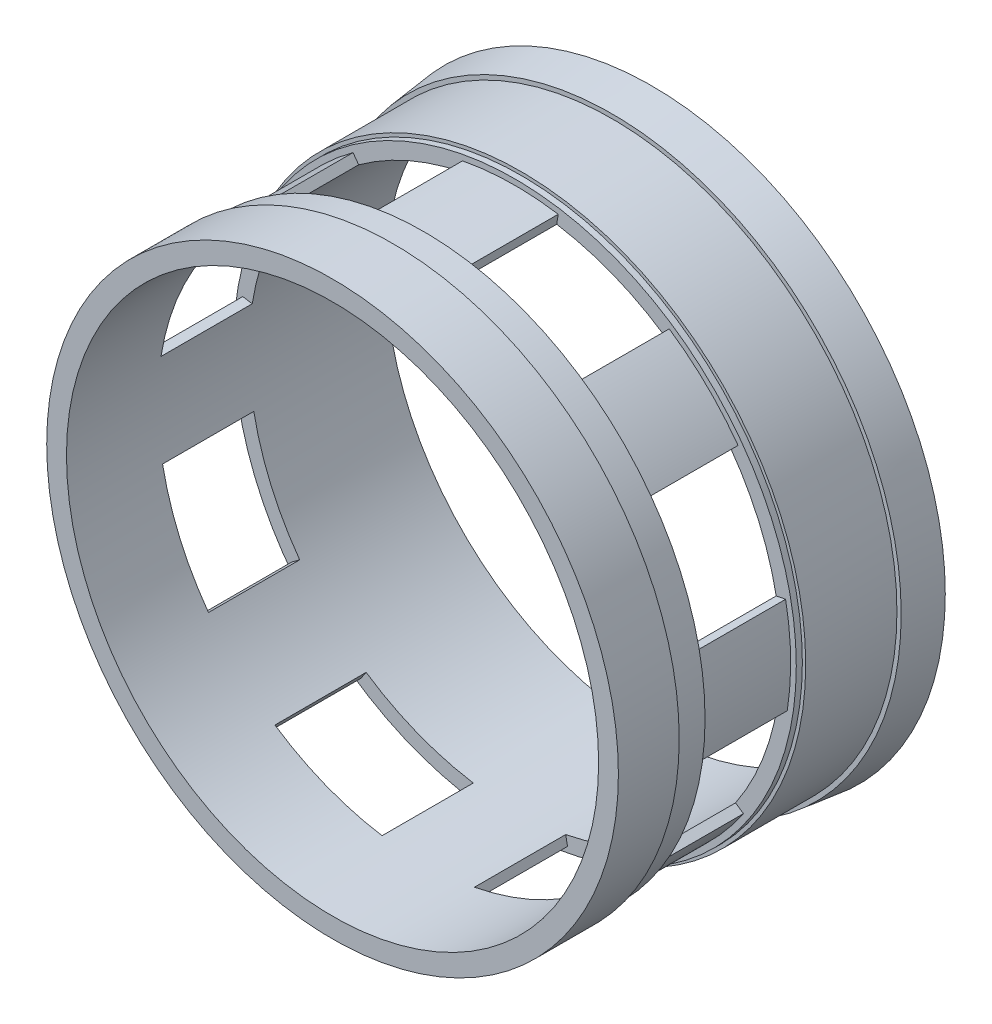
from build123d import *

# Parameters (mm, degrees)
SKETCH1_R           = 9.65
SKETCH2_R           = 9.5
SKETCH3_R           = 9.36
BOSS_EXTRUDE1_DEPTH = 3
SKETCH4_R           = 9.25
BOSS_EXTRUDE2_DEPTH = 0.2
SKETCH5_R           = 8.75
CUT_EXTRUDE1_DEPTH  = 10.2
BOSS_EXTRUDE3_START = 3
BOSS_EXTRUDE3_DEPTH = 3
CIRPATTERN1_COUNT   = 8
SKETCH8_R           = 9.25
BOSS_EXTRUDE4_DEPTH = 1
SKETCH9_R           = 9.4
BOSS_EXTRUDE5_DEPTH = 2
SKETCH11_R          = 8.75
CUT_EXTRUDE2_DEPTH  = 9


with BuildPart() as part:
    # Sketch1 → Loft2 section 0
    with BuildSketch(Plane.XY):
        Circle(SKETCH1_R)
    # Sketch2 → Loft2 section 1
    with BuildSketch(Plane.XY.offset(1.3)):
        Circle(SKETCH2_R)
    loft()

    # Sketch3 → Boss-Extrude1 (add)
    with BuildSketch(Plane.XY.offset(1.3)):
        Circle(SKETCH3_R)
    extrude(amount=BOSS_EXTRUDE1_DEPTH)

    # Sketch4 → Boss-Extrude2 (add)
    with BuildSketch(Plane.XY.offset(4.3)):
        Circle(SKETCH4_R)
    extrude(amount=BOSS_EXTRUDE2_DEPTH)

    # Sketch5 → Cut-Extrude1 (cut)
    with BuildSketch(Plane.XY.offset(4.5)):
        Circle(SKETCH5_R)
    extrude(amount=-CUT_EXTRUDE1_DEPTH, mode=Mode.SUBTRACT)

    # Sketch7 → Boss-Extrude3 (add)
    with BuildSketch(Plane.XY.offset(4.5).offset(BOSS_EXTRUDE3_START)):
        with BuildLine():
            Line((-1.666819903, 8.589773653), (-1.726800204, 8.898875558))
            ThreePointArc((-1.726800204, 8.898875558), (-0.155292705, 9.063537352), (1.420933285, 8.952808149))
            Line((1.420933285, 8.952808149), (1.371577253, 8.641832898))
            ThreePointArc((1.371577253, 8.641832898), (-0.149898622, 8.748715929), (-1.666819903, 8.589773653))
        make_face()
    boss_extrude3 = extrude(amount=-BOSS_EXTRUDE3_DEPTH)

    # CirPattern1: Boss-Extrude3 ×8 about axis
    cirpattern1_axis = Axis((0, 0, 0), (0, 0, 1))
    for i in range(1, CIRPATTERN1_COUNT):
        add(boss_extrude3.rotate(cirpattern1_axis, i * 360 / CIRPATTERN1_COUNT))

    # Sketch8 → Boss-Extrude4 (add)
    with BuildSketch(Plane.XY.offset(7.5)):
        Circle(SKETCH8_R)
    extrude(amount=BOSS_EXTRUDE4_DEPTH)

    # Sketch9 → Boss-Extrude5 (add)
    with BuildSketch(Plane.XY.offset(8.5)):
        Circle(SKETCH9_R)
    extrude(amount=BOSS_EXTRUDE5_DEPTH)

    # Sketch11 → Cut-Extrude2 (cut)
    with BuildSketch(Plane.XY.offset(10.5)):
        Circle(SKETCH11_R)
    extrude(amount=-CUT_EXTRUDE2_DEPTH, mode=Mode.SUBTRACT)


solid = part.part
